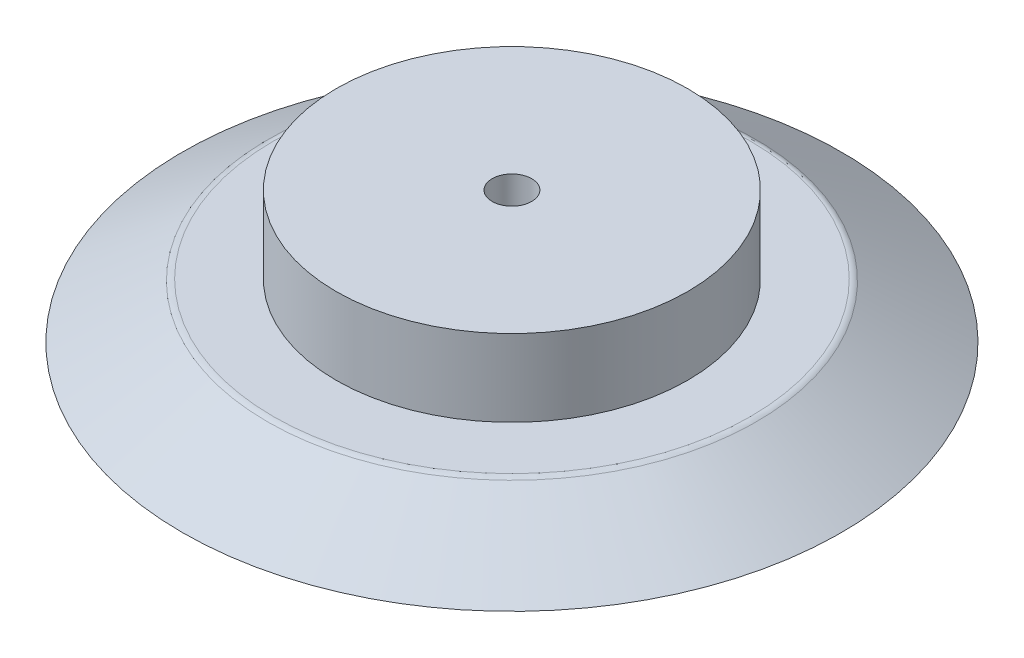
SolidWorks part; units mm, degrees
ref_plane "Front" through (0, 0, 0) normal (0, 0, 1) x (1, 0, 0)
ref_plane "Top" through (0, 0, 0) normal (0, 1, 0) x (1, 0, 0)
ref_plane "Side view" through (0, 0, 0) normal (1, 0, 0) x (0, 0, -1)
sketch "Sketch1" plane through (0, 0, 0) normal (0, 0, 1) x (1, 0, 0)
  line L0 (0, 20.8595) -> (0, -32.2041) construction
  line L1 (0, -15.4535) -> (-15, -15.4535)
  line L2 (-15, -15.4535) -> (-11.1216, -13.0295)
  line L3 (-8, -11.4535) -> (-8, -9.4535)
  line L4 (-8, -9.4535) -> (0, -9.4535)
  line L5 (0, -9.4535) -> (0, -15.4535)
  line L6 (-8, -11.4535) -> (-8, -12.9535)
  line L7 (-10.8566, -12.9535) -> (-8, -12.9535)
  arc A0 (-10.8566, -12.9535) -> (-11.1216, -13.0295) centre (-10.8566, -13.4535) ccw
  point P13 (-11, -12.9535)
  dimension "D7" = 0.5
  dimension "D1" = 15
  dimension "D3" = 7
  dimension "D4" = 6
  dimension "D5" = 2.5
  dimension "D6" = 11
revolve "Revolution1" add sketch "Sketch1" angle 360 about L0
hole_wizard "Clearance hole for M1.62" positions "Sketch9" profile "Sketch8" hole size "M1.6" standard "Ansi Metric" end condition through all
sketch "Sketch9" plane through (0, -15.4535, 0) normal (0, -1, 0) x (-1, 0, 0)
  point P0 (0, 0)
sketch "Sketch8" plane through (0, -15.4535, 0) normal (1, 0, 0) x (0, 0, -1)
  line L0 (0, 0) -> (0, 6)
  line L1 (0, 6) -> (0.9, 6)
  line L2 (0.9, 6) -> (0.9, 0)
  line L5 (0.9, 0) -> (0, 0)
  line L11 (0, -6.35) -> (0, 107.95) construction
  dimension "Diámetro de taladro hasta el siguiente" = 1.8
  dimension "Profundidad de taladro hasta el siguiente" = 6
